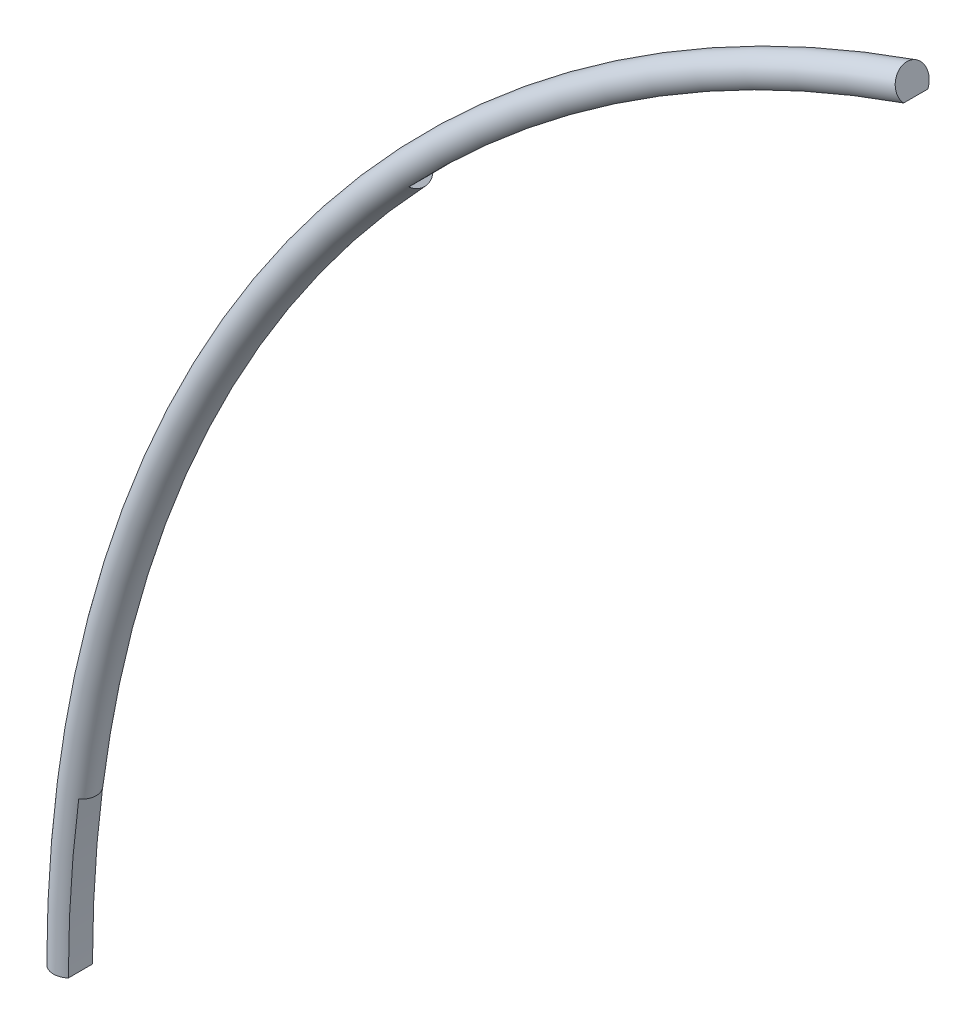
SolidWorks part; units mm, degrees
ref_plane "Front Plane" through (0, 0, 0) normal (0, 0, 1) x (1, 0, 0)
ref_plane "Top Plane" through (0, 0, 0) normal (0, 1, 0) x (1, 0, 0)
ref_plane "Right Plane" through (0, 0, 0) normal (1, 0, 0) x (0, 0, -1)
sketch "Sketch1" plane through (0, 0, 0) normal (0, 0, 1) x (1, 0, 0)
  line L0 (0, 0) -> (-121.3358, 0) construction
  line L1 (0, 0) -> (-36.7518, 105.5369) construction
  arc A0 (-76.6259, 220.0397) -> (-233, 0) centre (0, 0) ccw
  dimension "D1" = 70.8
  dimension "D2" = 233
sweep "Sweep1" add path "Sketch1" circular profile diameter 6 parameters "D3"=6
sketch "Sketch6" plane through (0, 0, 0) normal (0, 0, 1) x (1, 0, 0)
  line L0 (0, 0) -> (-231, 0)
  line L1 (0, 0) -> (-229.076, 29.7518)
  line L2 (0, 0) -> (-167.8387, 158.7172)
  line L3 (0, 0) -> (-75.9682, 218.1509)
  line L4 (-75.6393, 217.2066) -> (-77.6125, 222.8728) construction
  arc A0 (-75.9682, 218.1509) -> (-167.8387, 158.7172) centre (0, 0) ccw
  arc A1 (-229.076, 29.7518) -> (-231, 0) centre (0, 0) ccw
  dimension "D1" = 462
  dimension "D2" = 7.4
  dimension "D3" = 36
extrude "Cut-Extrude1" cut sketch "Sketch6" against normal mid plane 50 contours L1 A1 L0 | L3 A0 L2
